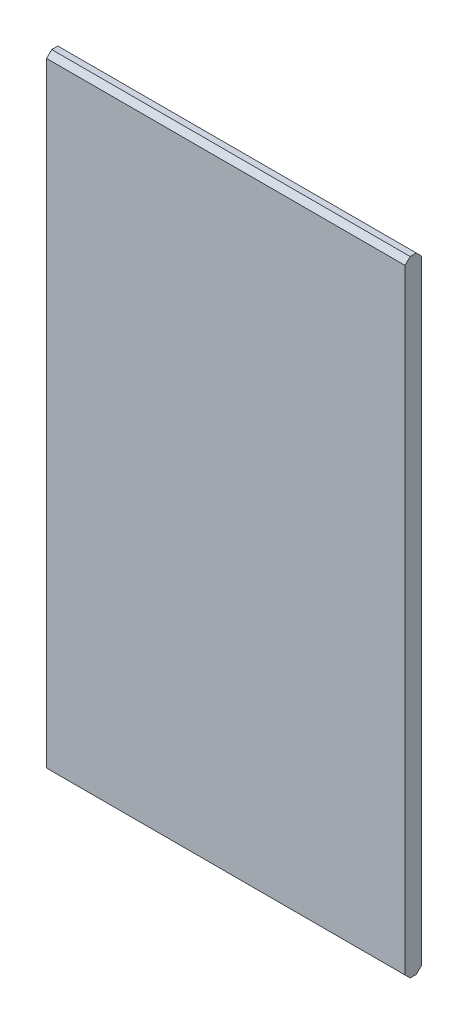
SolidWorks part; units mm, degrees
ref_plane "Front Plane" through (0, 0, 0) normal (0, 0, 1) x (1, 0, 0)
ref_plane "Top Plane" through (0, 0, 0) normal (0, 1, 0) x (1, 0, 0)
ref_plane "Right Plane" through (0, 0, 0) normal (1, 0, 0) x (0, 0, -1)
sketch "Sketch1" plane through (0, 0, 0) normal (0, 0, 1) x (1, 0, 0)
  line L1 (0, 0) -> (350, 0)
  line L2 (0, 0) -> (0, 610)
  line L3 (0, 610) -> (350, 610)
  line L4 (350, 0) -> (350, 610)
  dimension "D1" = 350
  dimension "D2" = 610
extrude "Boss-Extrude1" add sketch "Sketch1" along normal blind 16
chamfer "Chamfer1" distance 5 angle 45 5 edges at (0, 305, 16) (175, 610, 0) (175, 610, 16) (175, 0, 0) (175, 0, 16)
